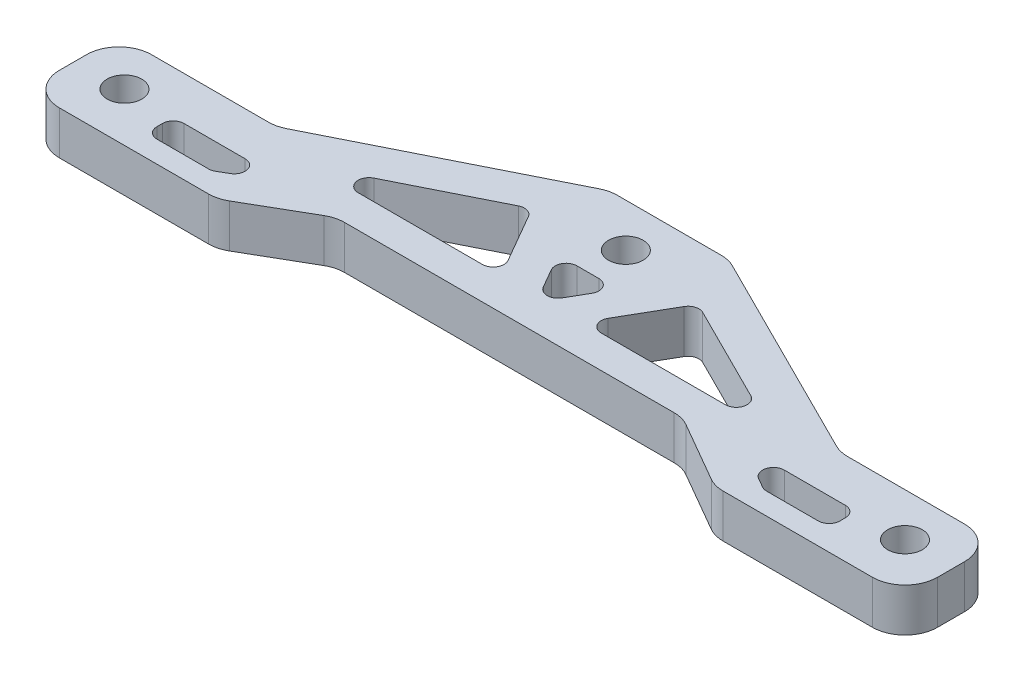
SolidWorks part; units mm, degrees
material "Thornel Mat VMA"
ref_plane "前视基准面" through (0, 0, 0) normal (0, 0, 1) x (1, 0, 0)
ref_plane "上视基准面" through (0, 0, 0) normal (0, 1, 0) x (1, 0, 0)
ref_plane "右视基准面" through (0, 0, 0) normal (1, 0, 0) x (0, 0, -1)
sketch "草图1" plane through (0, 0, 0) normal (0, 1, 0) x (1, 0, 0)
  line L0 (-36, 0) -> (36, 0) construction
  line L1 (0, 10.25) -> (0, 0) construction
  line L2 (-40.5, -4.5) -> (-22.9282, -4.5)
  line L3 (40.5, -4.5) -> (40.5, 4)
  line L4 (40.5, 4) -> (26, 4)
  line L6 (5.5, 14.25) -> (-5.5, 14.25)
  line L7 (-40.5, -4.5) -> (-40.5, 4)
  line L8 (-40.5, 4) -> (-26, 4)
  line L10 (-22.9282, -4.5) -> (-16, -0.5)
  line L11 (-16, -0.5) -> (16, -0.5)
  line L12 (16, -0.5) -> (22.9282, -4.5)
  line L13 (22.9282, -4.5) -> (40.5, -4.5)
  line L14 (-26, 4) -> (-5.5, 14.25)
  line L15 (26, 4) -> (5.5, 14.25)
  circle A0 centre (-36, 0) radius 1.6
  circle A1 centre (36, 0) radius 1.6
  circle A2 centre (0, 10.25) radius 1.6
  dimension "D1" = 10.25
  dimension "D2" = 3.2
  dimension "D3" = 72
  dimension "D4" = 4
  dimension "D5" = 4.5
  dimension "D6" = 4.5
  dimension "D7" = 10
  dimension "D8" = 150
  dimension "D9" = 0.5
  dimension "D10" = 32
  dimension "D11" = 4
  dimension "D12" = 11
extrude "凸台-拉伸1" add sketch "草图1" along normal blind 4
sketch "草图2" plane through (0, 4, 0) normal (0, 1, 0) x (1, 0, 0)
  line L0 (-36, 0) -> (0, 10.25) construction
  line L1 (0, 10.25) -> (36, 0) construction
  line L2 (-7.6552, 9.2593) -> (-21.1738, 2.5)
  line L3 (-21.1738, 2.5) -> (-3.7528, 2.5)
  line L4 (-3.7528, 2.5) -> (-7.6552, 9.2593)
  line L5 (-2.7424, 6.75) -> (0, 2)
  line L6 (-2.7424, 6.75) -> (2.7424, 6.75)
  line L7 (2.7424, 6.75) -> (0, 2)
  line L8 (0, 10.25) -> (0, 0) construction
  line L9 (21.1738, 2.5) -> (3.7528, 2.5)
  line L10 (7.6552, 9.2593) -> (21.1738, 2.5)
  line L11 (3.7528, 2.5) -> (7.6552, 9.2593)
  line L12 (-5.5, 14.25) -> (-26, 4) construction
  line L13 (-16, -0.5) -> (16, -0.5) construction
  line L14 (-31.5, 0) -> (-21.134, 0)
  line L15 (-21.134, 0) -> (-25.4641, -2.5)
  line L16 (-25.4641, -2.5) -> (-31.5, -2.5)
  line L17 (-31.5, -2.5) -> (-31.5, 0)
  line L18 (25.4641, -2.5) -> (31.5, -2.5)
  line L19 (21.134, 0) -> (25.4641, -2.5)
  line L20 (31.5, 0) -> (21.134, 0)
  line L21 (31.5, -2.5) -> (31.5, 0)
  line L22 (-40.5, -4.5) -> (-22.9282, -4.5) construction
  line L23 (-22.9282, -4.5) -> (-16, -0.5) construction
  dimension "D1" = 3.5
  dimension "D2" = 3
  dimension "D3" = 3.5
  dimension "D4" = 2.5
  dimension "D5" = 3
  dimension "D6" = 60
  dimension "D7" = 2.5
  dimension "D8" = 2
  dimension "D9" = 4.5
  dimension "D10" = 3
extrude "切除-拉伸1" cut sketch "草图2" against normal through all
fillet "R1 镂空圆角" radius 1 17 edges at (21.1738, 2, -2.5) (3.7528, 2, -2.5) (7.6552, 2, -9.2593) (2.7424, 2, -6.75) (0, 2, -2) (-2.7424, 2, -6.75) (-3.7528, 2, -2.5) (-21.1738, 2, -2.5) (-7.6552, 2, -9.2593) (21.134, 2, 0) (31.5, 2, 2.5) (25.4641, 2, 2.5) (31.5, 2, 0) (-31.5, 2, 2.5) (-21.134, 2, 0) (-25.4641, 2, 2.5) (-31.5, 2, 0)
fillet "R3 外缘圆角" radius 3 12 edges at (40.5, 2, -4) (40.5, 2, 4.5) (22.9282, 2, 4.5) (16, 2, 0.5) (-16, 2, 0.5) (-22.9282, 2, 4.5) (-40.5, 2, -4) (-26, 2, -4) (-5.5, 2, -14.25) (5.5, 2, -14.25) (26, 2, -4) (-40.5, 2, 4.5)
